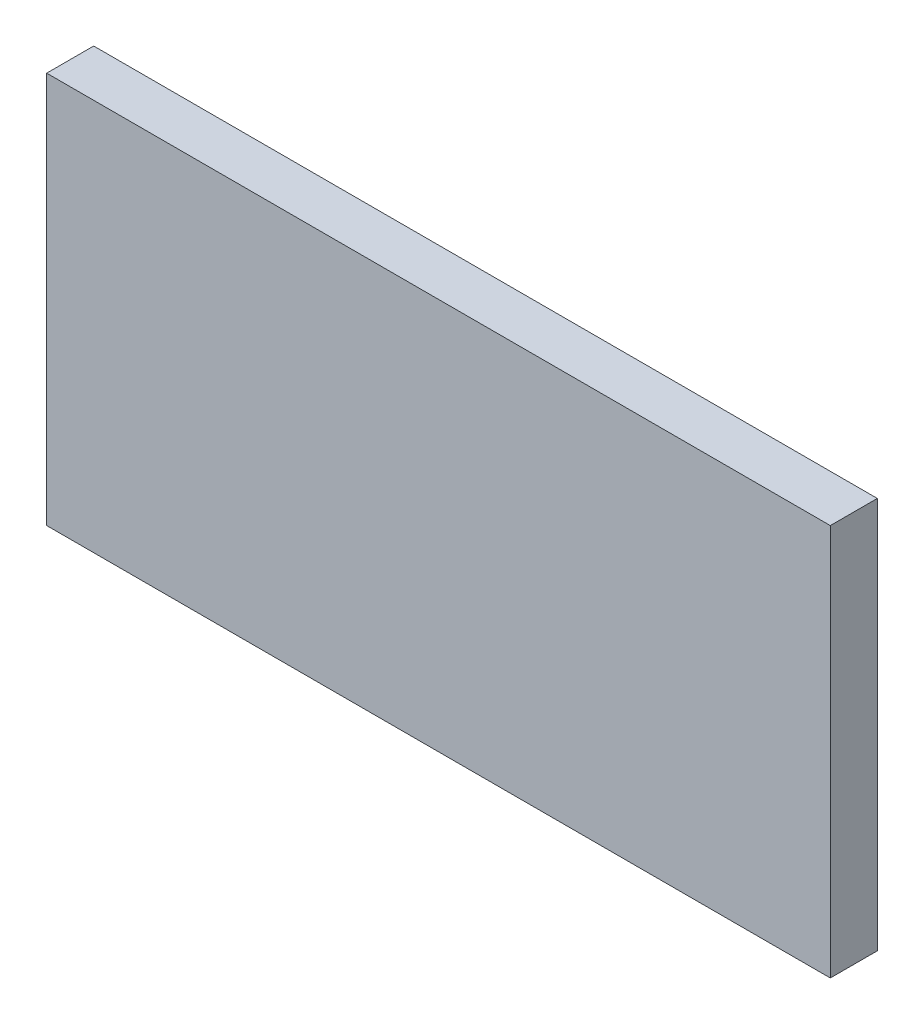
SolidWorks part; units mm, degrees
ref_plane "前视基准面" through (0, 0, 0) normal (0, 0, 1) x (1, 0, 0)
ref_plane "上视基准面" through (0, 0, 0) normal (0, 1, 0) x (1, 0, 0)
ref_plane "右视基准面" through (0, 0, 0) normal (1, 0, 0) x (0, 0, -1)
sketch "草图1" plane through (0, 0, 0) normal (0, 0, 1) x (1, 0, 0)
  line L1 (-100, -50) -> (100, -50)
  line L2 (-100, -50) -> (-100, 50)
  line L3 (-100, 50) -> (100, 50)
  line L4 (100, -50) -> (100, 50)
  line L5 (-100, -50) -> (100, 50) construction
  line L6 (-100, 50) -> (100, -50) construction
  point P0 (0, 0)
  dimension "D1" = 200
  dimension "D2" = 100
extrude "凸台-拉伸1" add sketch "草图1" along normal blind 12
